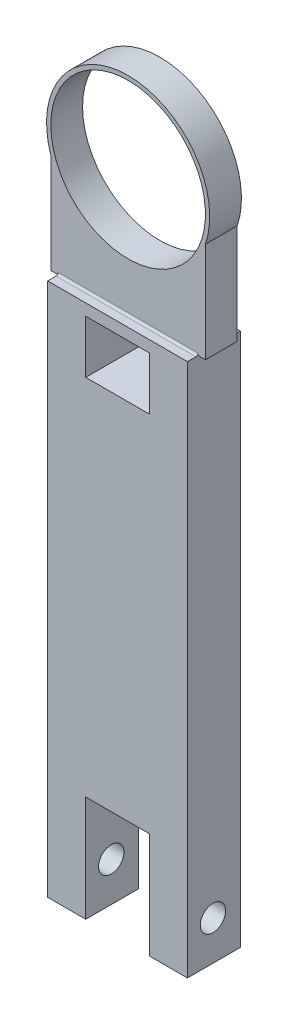
from build123d import *
from build123d.topology import SkipClean

# Parameters (mm, degrees)
EXTRUDE_1_DEPTH          = 12.5
HOLE_WIZARD_M14_1_D      = 12
HOLE_WIZARD_M14_1_DEPTH  = 18
SKETCH_7_W               = 66
SKETCH_7_H               = 25
EXTRUDE_2_DEPTH          = 12
CUT_EXTRUDE_1_DEPTH      = 156.608483059
CUT_EXTRUDE_1_DEPTH_BACK = 156.608483059
SKETCH_14_W              = 30
SKETCH_14_H              = 25
EXTRUDE_START            = -12.5
EXTRUDE_3_DEPTH          = 7.5
SKETCH_8_4_R             = 38.5
SKETCH_8_4_R_2           = 36.5
EXTRUDE_1_2_DEPTH        = 7.5
FILLET_1_R               = 1


with BuildPart() as part:
    # 草图1 → Extrude 1 (new, symmetric)
    with BuildSketch(Plane.XY):
        Polygon((-33, -150), (-15, -150), (-15, -100), (0, -100), (15, -100), (15, -150), (33, -150), (33, 90), (15, 90), (-15, 90), (-33, 90), align=None)
    extrude(amount=EXTRUDE_1_DEPTH, both=True)

    # M14 螺纹孔1
    with Locations(Plane(origin=(33, -131.5, 0.451602972), x_dir=(0, 0, 1), z_dir=(1, 0, 0))):
        with Locations((0, 0)):
            hole_wizard_m14_1 = Hole(HOLE_WIZARD_M14_1_D / 2, depth=HOLE_WIZARD_M14_1_DEPTH)

    # 镜向1: M14 螺纹孔1 across plane
    add(hole_wizard_m14_1.mirror(Plane(origin=(0, 0, 0), x_dir=(0, 0, 1), z_dir=(1, 0, 0))), mode=Mode.SUBTRACT)

    # 草图7 → 凸台-拉伸2 (add)
    with BuildSketch(Plane(origin=(0, 90, 0), x_dir=(1, 0, 0), z_dir=(0, 1, 0))):
        Rectangle(SKETCH_7_W, SKETCH_7_H)
    extrude(amount=EXTRUDE_2_DEPTH)

    # 草图14 → 切除-拉伸1 (cut, two sides: drawn at the far end of the back side and taken through both)
    with BuildSketch(Plane(origin=(0, 0, -12.5), x_dir=(-1, 0, 0), z_dir=(0, 0, -1)).offset(-CUT_EXTRUDE_1_DEPTH_BACK)):
        with Locations((0, 84.064537633)):
            Rectangle(SKETCH_14_W, SKETCH_14_H)
    extrude(amount=CUT_EXTRUDE_1_DEPTH + CUT_EXTRUDE_1_DEPTH_BACK, mode=Mode.SUBTRACT)

    # 草图8 → 凸台-拉伸3 (add, symmetric)
    with BuildSketch(Plane(origin=(0, 0, -12.5), x_dir=(-1, 0, 0), z_dir=(0, 0, -1)).offset(EXTRUDE_START)):
        with BuildLine():
            Line((-33, 102), (0, 102))
            Line((0, 102), (0, 125))
            ThreePointArc((0, 125), (-25.809397513, 135.690602487), (-36.5, 161.5))
            Line((-36.5, 161.5), (-36.5, 102))
            Line((-36.5, 102), (-33, 102))
        make_face()
        with BuildLine():
            Line((0, 102), (33, 102))
            Line((33, 102), (36.5, 102))
            Line((36.5, 102), (36.5, 161.5))
            ThreePointArc((36.5, 161.5), (25.809397513, 135.690602487), (0, 125))
            Line((0, 125), (0, 102))
        make_face()
    extrude(amount=EXTRUDE_3_DEPTH, both=True)

    # 草图8<4> → Extrude 1 2 (add, symmetric)
    with SkipClean():  # the faces are left unmerged after this step: merging them gives an invalid solid
        with BuildSketch(Plane(origin=(0, 0, -12.5), x_dir=(-1, 0, 0), z_dir=(0, 0, -1)).offset(EXTRUDE_START)):
            with Locations((0, 161.5)):
                Circle(SKETCH_8_4_R)
            with Locations((0, 161.5)):
                Circle(SKETCH_8_4_R_2, mode=Mode.SUBTRACT)
        extrude(amount=EXTRUDE_1_2_DEPTH, both=True)

    # 圆角1
    fillet_1_edges = [part.edges().sort_by_distance(p)[0] for p in [
        (0, 102, -7.5),
        (0, 102, 7.5),
    ]]
    fillet(fillet_1_edges, radius=FILLET_1_R)


solid = part.part
